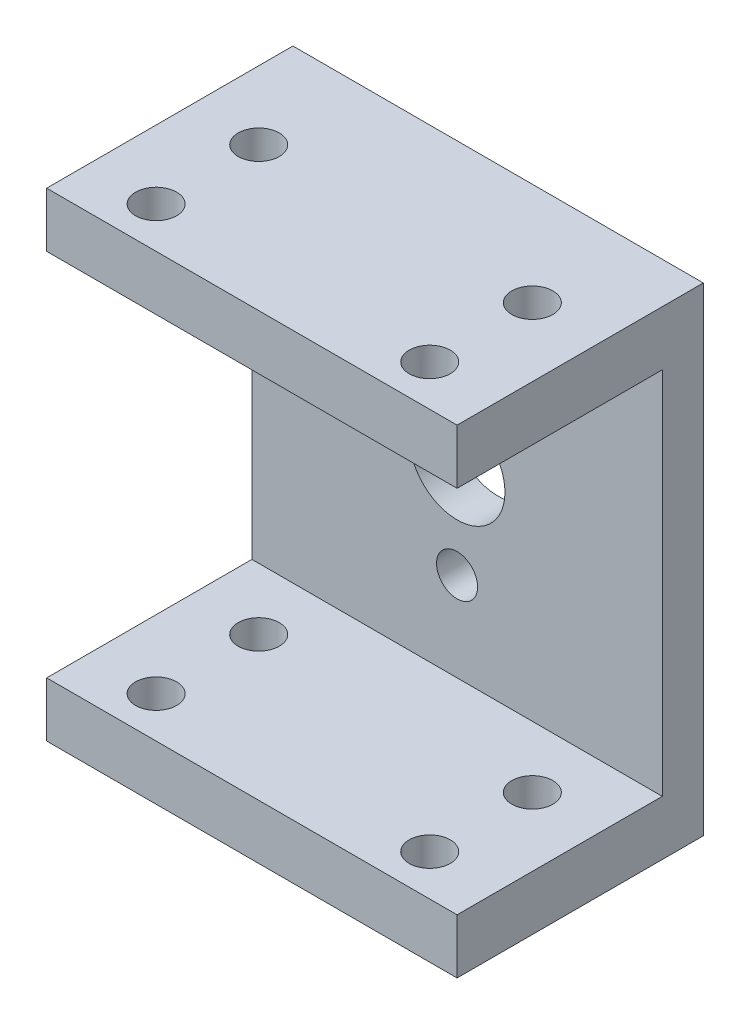
from build123d import *

# Parameters (mm, degrees)
SKETCH1_W           = 30
SKETCH1_H           = 35
SKETCH1_R           = 3.5
SKETCH1_R_2         = 1.5
BOSS_EXTRUDE1_DEPTH = 3
SKETCH2_W           = 30
SKETCH2_H           = 4
BOSS_EXTRUDE2_DEPTH = 15
SKETCH4_R           = 1.5
CUT_EXTRUDE1_DEPTH  = 15


with BuildPart() as part:
    # Sketch1 → Boss-Extrude1 (new body)
    with BuildSketch(Plane.XY):
        Rectangle(SKETCH1_W, SKETCH1_H)
        Circle(SKETCH1_R, mode=Mode.SUBTRACT)
        with Locations((0, 7)):
            Circle(SKETCH1_R_2, mode=Mode.SUBTRACT)
        with Locations(Location((0, -7, 0), (0, 0, 180))):
            Circle(SKETCH1_R_2, mode=Mode.SUBTRACT)
    extrude(amount=BOSS_EXTRUDE1_DEPTH)

    # Sketch2 → Boss-Extrude2 (add)
    with BuildSketch(Plane.XY.offset(3)):
        with Locations((0, 15.5)):
            Rectangle(SKETCH2_W, SKETCH2_H)
        with Locations((0, -15.5)):
            Rectangle(SKETCH2_W, SKETCH2_H)
    extrude(amount=BOSS_EXTRUDE2_DEPTH)

    # Sketch4 → Cut-Extrude1 (cut)
    with BuildSketch(Plane.XZ.offset(-13.5)):
        with Locations(Location((-10, 15, 0), (0, 0, 270))):
            Circle(SKETCH4_R)
        with Locations(Location((10, 15, 0), (0, 0, 270))):
            Circle(SKETCH4_R)
        with Locations(Location((10, 7.5, 0), (0, 0, 270))):
            Circle(SKETCH4_R)
        with Locations(Location((-10, 7.5, 0), (0, 0, 270))):
            Circle(SKETCH4_R)
    cut_extrude1 = extrude(amount=-CUT_EXTRUDE1_DEPTH, mode=Mode.SUBTRACT)

    # Mirror1: Cut-Extrude1 across plane
    add(cut_extrude1.mirror(Plane.ZX), mode=Mode.SUBTRACT)


solid = part.part
